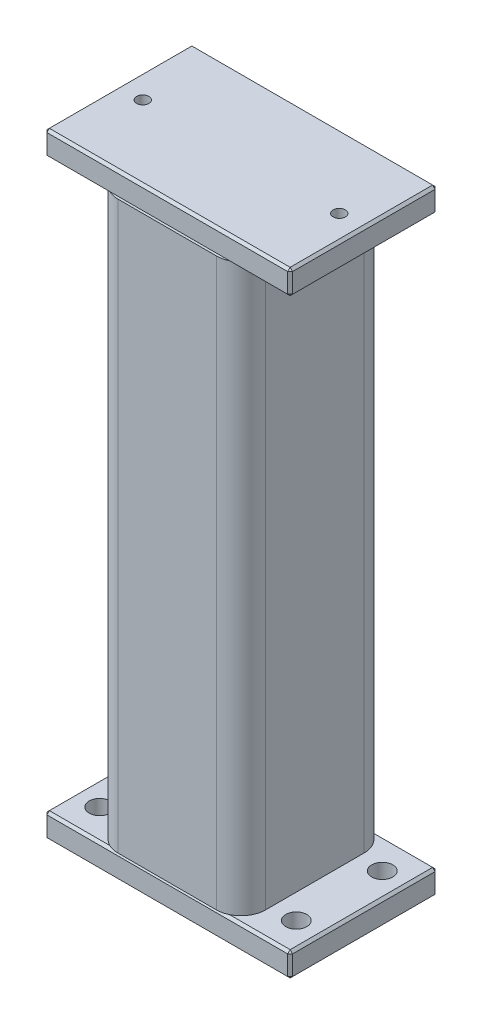
SolidWorks part; units mm, degrees
material "45号钢"
ref_plane "Front" through (0, 0, 0) normal (0, 0, 1) x (1, 0, 0)
ref_plane "Top" through (0, 0, 0) normal (0, 1, 0) x (1, 0, 0)
ref_plane "Right" through (0, 0, 0) normal (1, 0, 0) x (0, 0, -1)
sketch3d "3D草图1"
  line L0 (0, 0, 0) -> (0, 230.5, 0)
  dimension "D1" = 230.5
other "结构构件1"
ref_plane "基准面1" through (0, 0, 0) normal (0, 1, 0) x (1, 0, 0)
sketch "Sketch11" plane through (0, 0, 0) normal (0, 1, 0) x (1, 0, 0)
  line L0 (-20, -25) -> (20, -25)
  line L1 (-25, -20) -> (-25, 20)
  line L2 (20, 25) -> (-20, 25)
  line L3 (25, 20) -> (25, -20)
  line L4 (-20, -30) -> (20, -30)
  line L5 (-30, -20) -> (-30, 20)
  line L6 (20, 30) -> (-20, 30)
  line L7 (30, 20) -> (30, -20)
  arc A0 (30, 20) -> (20, 30) centre (20, 20) ccw
  arc A1 (20, -30) -> (30, -20) centre (20, -20) ccw
  arc A2 (-30, -20) -> (-20, -30) centre (-20, -20) ccw
  arc A3 (-20, 30) -> (-30, 20) centre (-20, 20) ccw
  arc A4 (-20, 25) -> (-25, 20) centre (-20, 20) ccw
  arc A5 (25, 20) -> (20, 25) centre (20, 20) ccw
  arc A6 (20, -25) -> (25, -20) centre (20, -20) ccw
  arc A7 (-25, -20) -> (-20, -25) centre (-20, -20) ccw
  point P0 (-30, 0)
  point P1 (30, 0)
  point P2 (0, 30)
  point P3 (0, -30)
  point P4 (0, 0)
  point P5 (-30, -30)
  point P6 (30, -30)
  point P7 (30, 30)
  point P8 (-30, 30)
  point P33 (0, 0)
  dimension "D1" = 10
  dimension "D2" = 60
  dimension "D3" = 5
sketch "草图2" plane through (0, 230.5, 0) normal (0, 1, 0) x (1, 0, 0)
  line L0 (20, 30) -> (-20, 30) construction
  line L1 (-50, 30) -> (50, 30)
  line L2 (-50, 30) -> (-50, -30)
  line L3 (-50, -30) -> (50, -30)
  line L4 (50, 30) -> (50, -30)
  line L5 (-50, 30) -> (50, -30) construction
  line L6 (-50, -30) -> (50, 30) construction
  point P0 (0, 0)
  dimension "D1" = 100
extrude "凸台-拉伸1" add sketch "草图2" along normal blind 10 separate body
sketch "草图3" plane through (0, 0, 0) normal (0, -1, 0) x (1, 0, 0)
  line L0 (-20, 30) -> (20, 30) construction
  line L1 (-50, 30) -> (50, 30)
  line L2 (-50, 30) -> (-50, -30)
  line L3 (-50, -30) -> (50, -30)
  line L4 (50, 30) -> (50, -30)
  line L5 (-50, 30) -> (50, -30) construction
  line L6 (-50, -30) -> (50, 30) construction
  line L7 (30, 20) -> (30, -20) construction
  point P0 (0, 0)
  dimension "D1" = 20
extrude "凸台-拉伸2" add sketch "草图3" along normal blind 10 separate body
chamfer "倒角1" distance 1 angle 45 12 edges at (0, 240.5, -30) (0, 230.5, -30) (50, 240.5, 0) (50, 235.5, -30) (50, 230.5, 0) (-50, 235.5, -30) (-50, 240.5, 0) (-50, 230.5, 0) (-50, 235.5, 30) (0, 240.5, 30) (50, 235.5, 30) (0, 230.5, 30)
chamfer "倒角2" distance 1 angle 45 12 edges at (-50, -10, 0) (-50, 0, 0) (-50, -5, -30) (0, -10, -30) (0, 0, -30) (0, -10, 30) (-50, -5, 30) (0, 0, 30) (50, -5, -30) (50, -10, 0) (50, -5, 30) (50, 0, 0)
hole_wizard "Ø8.6 (8.6) 直径孔1" positions "草图5" profile "草图4" hole size "Ø8.6" standard "Ansi Metric"
sketch "草图5" plane through (0, 0, 0) normal (0, 1, 0) x (1, 0, 0)
  line L0 (0, 0) -> (0, -30) construction
  line L1 (49, -30) -> (-49, -30) construction
  line L3 (0, 0) -> (50, 0) construction
  line L4 (50, 29) -> (50, -29) construction
  point P0 (40, 17.5)
  point P2 (40, -17.5)
  point P4 (-40, 17.5)
  point P6 (-40, -17.5)
  dimension "D1" = 80
  dimension "D2" = 35
sketch "草图4" plane through (40, 0, -17.5) normal (1, 0, 0) x (0, 0, 1)
  line L0 (0, 0) -> (0, 18.0926)
  line L1 (0, 18.0926) -> (4.3, 15.61)
  line L2 (4.3, 15.61) -> (4.3, 0)
  line L5 (4.3, 0) -> (0, 0)
  line L10 (0, 18.0926) -> (-4.3, 15.61) construction
  line L11 (0, -6.35) -> (0, 107.95) construction
  dimension "孔直径" = 8.6
  dimension "孔深度" = 15.61
  dimension "导头角度" = 120
sketch "草图6" plane through (0, 0, 0) normal (0, 1, 0) x (1, 0, 0)
  line L0 (-40, -17.5) -> (-40, 17.5) construction
  line L1 (40, -17.5) -> (40, 17.5) construction
  circle A0 centre (-40, 0) radius 4
  circle A1 centre (40, 0) radius 4
  dimension "D1" = 8
hole_wizard "M6 螺纹孔1" positions "草图12" profile "草图11" tap size "M6" standard "Gb"
sketch "草图12" plane through (0, 240.5, 0) normal (0, 1, 0) x (1, 0, 0)
  point P0 (-40, 0)
  point P3 (40, 0)
sketch "草图11" plane through (-40, 240.5, 0) normal (1, 0, 0) x (0, 0, 1)
  line L0 (0, 0) -> (0, 18.5022)
  line L1 (0, 18.5022) -> (2.5, 17)
  line L2 (2.5, 17) -> (2.5, 0)
  line L5 (2.5, 0) -> (0, 0)
  line L10 (0, 18.5022) -> (-2.5, 17) construction
  line L11 (0, -6.35) -> (0, 107.95) construction
  dimension "螺纹孔钻头直径" = 5
  dimension "螺纹孔钻头深度" = 17
  dimension "导头角度" = 118
cosmetic thread "孔螺蚊线1" parameters "D1"=10, "D2"=6
cosmetic thread "孔螺蚊线2" parameters "D1"=10, "D2"=6
